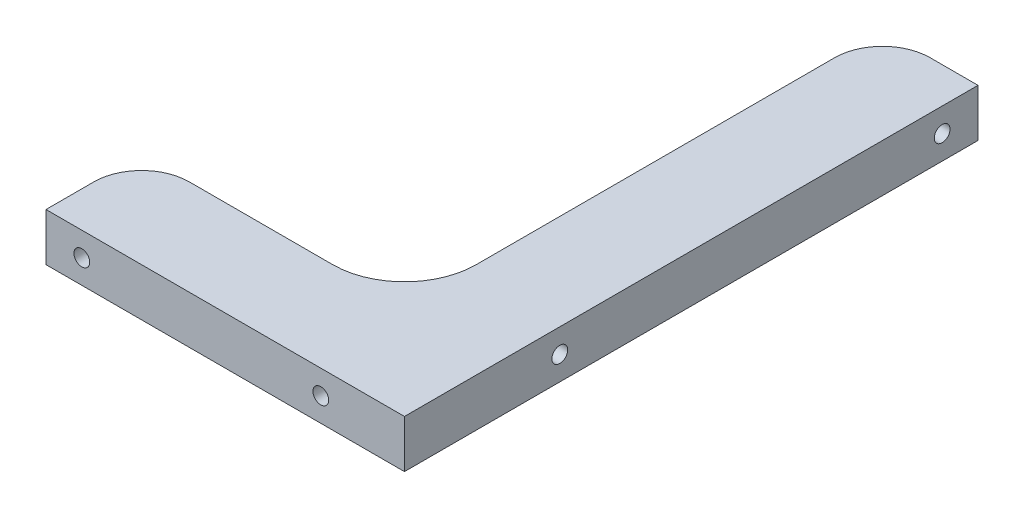
from build123d import *

# Parameters (mm, degrees)
SKETCH_1_W             = 75
SKETCH_1_H             = 120
EXTRUDE_1_DEPTH        = 5
SKETCH_2_W             = 55
SKETCH_2_H             = 100
CUT_EXTRUDE_1_DEPTH    = 10
FILLET_1_R             = 15
FILLET_2_R             = 10
HOLE_WIZARD_M4_1_D     = 3.3
HOLE_WIZARD_M4_1_DEPTH = 10.1
HOLE_WIZARD_M4_1_TIP   = 0.991420021
HOLE_WIZARD_M4_2_D     = 3.3
HOLE_WIZARD_M4_2_DEPTH = 10.1
HOLE_WIZARD_M4_2_TIP   = 0.991420021


with BuildPart() as part:
    # 草图1 → 凸台-拉伸1 (new, symmetric)
    with BuildSketch(Plane(origin=(0, 0, 0), x_dir=(1, 0, 0), z_dir=(0, 1, 0))):
        Rectangle(SKETCH_1_W, SKETCH_1_H)
    extrude(amount=EXTRUDE_1_DEPTH, both=True)

    # 草图2 → 切除-拉伸1 (cut)
    with BuildSketch(Plane(origin=(0, 5, 0), x_dir=(1, 0, 0), z_dir=(0, 1, 0))):
        with Locations((-10, 10)):
            Rectangle(SKETCH_2_W, SKETCH_2_H)
    extrude(amount=-CUT_EXTRUDE_1_DEPTH, mode=Mode.SUBTRACT)

    # 圆角1
    fillet_1_edges = [part.edges().sort_by_distance(p)[0] for p in [
        (17.5, 0, 40),
    ]]
    fillet(fillet_1_edges, radius=FILLET_1_R)

    # 圆角2
    fillet_2_edges = [part.edges().sort_by_distance(p)[0] for p in [
        (17.5, 0, -60),
        (-37.5, 0, 40),
    ]]
    fillet(fillet_2_edges, radius=FILLET_2_R)

    # M4 螺纹孔1
    with Locations(Plane.XY.offset(60)):
        with Locations((-30, 0), (20, 0)):
            Hole(HOLE_WIZARD_M4_1_D / 2, depth=HOLE_WIZARD_M4_1_DEPTH)
            with Locations((0, 0, -(HOLE_WIZARD_M4_1_DEPTH + HOLE_WIZARD_M4_1_TIP / 2))):  # 118° drill point
                Cone(0, HOLE_WIZARD_M4_1_D / 2, HOLE_WIZARD_M4_1_TIP, mode=Mode.SUBTRACT)

    # M4 螺纹孔2
    with Locations(Plane(origin=(37.5, 0, 0), x_dir=(0, 0, -1), z_dir=(1, 0, 0))):
        with Locations((-27.5, 0), (52.5, 0)):
            Hole(HOLE_WIZARD_M4_2_D / 2, depth=HOLE_WIZARD_M4_2_DEPTH)
            with Locations((0, 0, -(HOLE_WIZARD_M4_2_DEPTH + HOLE_WIZARD_M4_2_TIP / 2))):  # 118° drill point
                Cone(0, HOLE_WIZARD_M4_2_D / 2, HOLE_WIZARD_M4_2_TIP, mode=Mode.SUBTRACT)


solid = part.part
